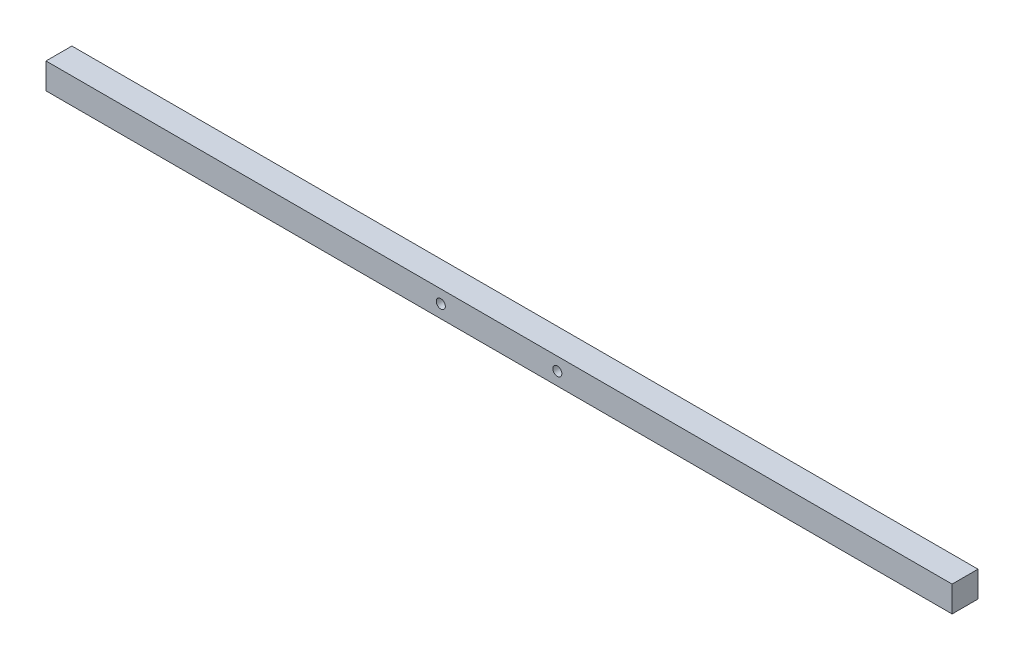
from build123d import *

# Parameters (mm, degrees)
SKETCH_1_W          = 20
SKETCH_1_H          = 20
EXTRUDE_1_DEPTH     = 350
SKETCH_2_R          = 3.5
CUT_EXTRUDE_1_DEPTH = 700


with BuildPart() as part:
    # 草图1 → 凸台-拉伸1 (new, symmetric)
    with BuildSketch(Plane(origin=(0, 0, 0), x_dir=(0, 0, -1), z_dir=(1, 0, 0))):
        Rectangle(SKETCH_1_W, SKETCH_1_H)
    extrude(amount=EXTRUDE_1_DEPTH, both=True)

    # 草图2 → 切除-拉伸1 (cut)
    with BuildSketch(Plane.XY.offset(10)):
        with Locations((-45, 0)):
            Circle(SKETCH_2_R)
        with Locations((45, 0)):
            Circle(SKETCH_2_R)
    extrude(amount=-CUT_EXTRUDE_1_DEPTH, mode=Mode.SUBTRACT)


solid = part.part
